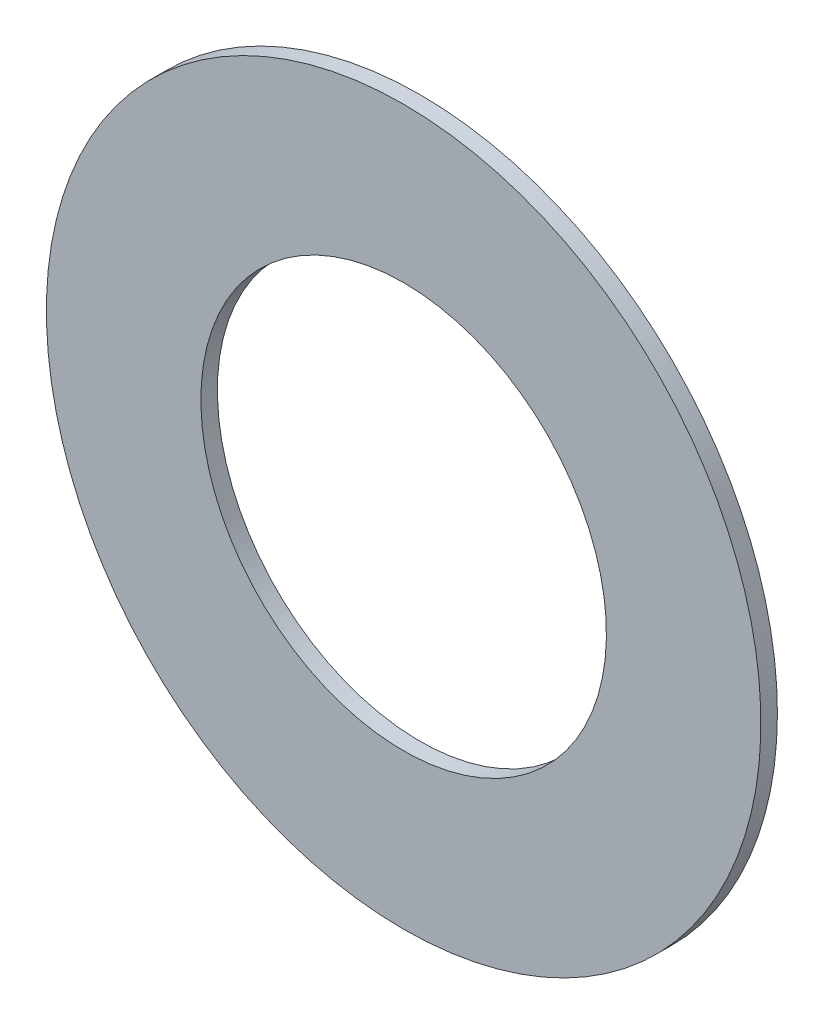
SolidWorks part; units mm, degrees
material "Brass"
ref_plane "Front" through (0, 0, 0) normal (0, 0, 1) x (1, 0, 0)
ref_plane "Top" through (0, 0, 0) normal (0, 1, 0) x (1, 0, 0)
ref_plane "Right" through (0, 0, 0) normal (1, 0, 0) x (0, 0, -1)
sketch "Sketch1" plane through (0, 0, 0) normal (0, 0, 1) x (1, 0, 0)
  circle A1 centre (0, 0) radius 37
  circle A3 centre (0, 0) radius 21
extrude "Boss-Extrude1" add sketch "Sketch1" along normal up to surface (1.71 mm away) contours A1
